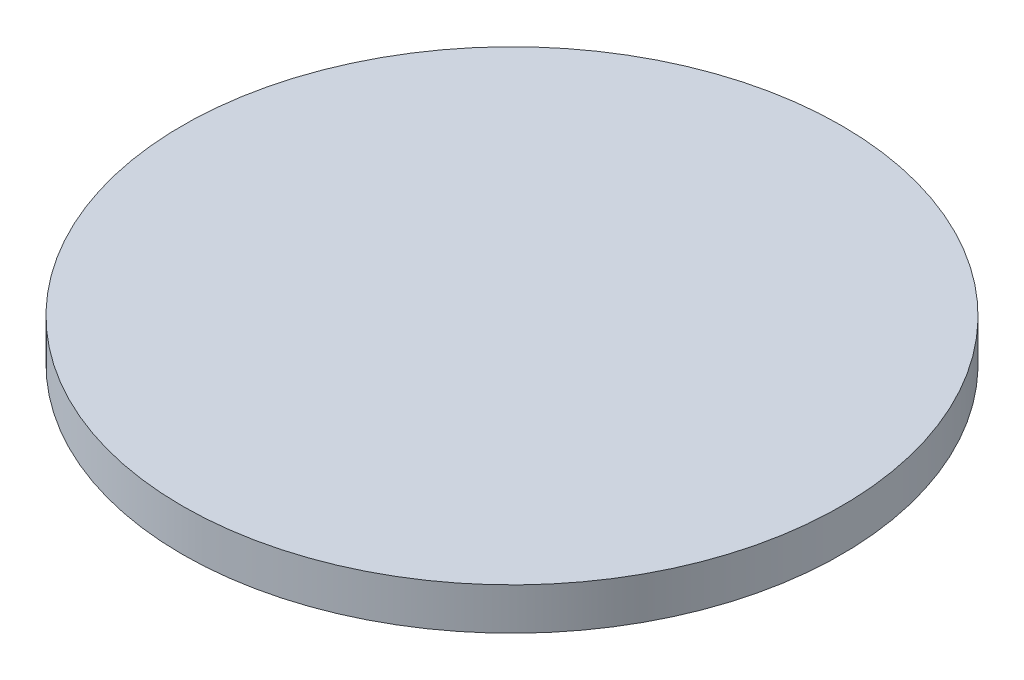
from build123d import *

# Parameters (mm, degrees)
SKETCH1_R           = 11.8
BOSS_EXTRUDE1_DEPTH = 1.5


with BuildPart() as part:
    # Sketch1 → Boss-Extrude1 (new body)
    with BuildSketch(Plane(origin=(0, 210, 0), x_dir=(1, 0, 0), z_dir=(0, 1, 0))):
        with Locations(Location((0, 0, 0), (0, 0, 270))):
            Circle(SKETCH1_R)
    extrude(amount=-BOSS_EXTRUDE1_DEPTH)


solid = part.part
